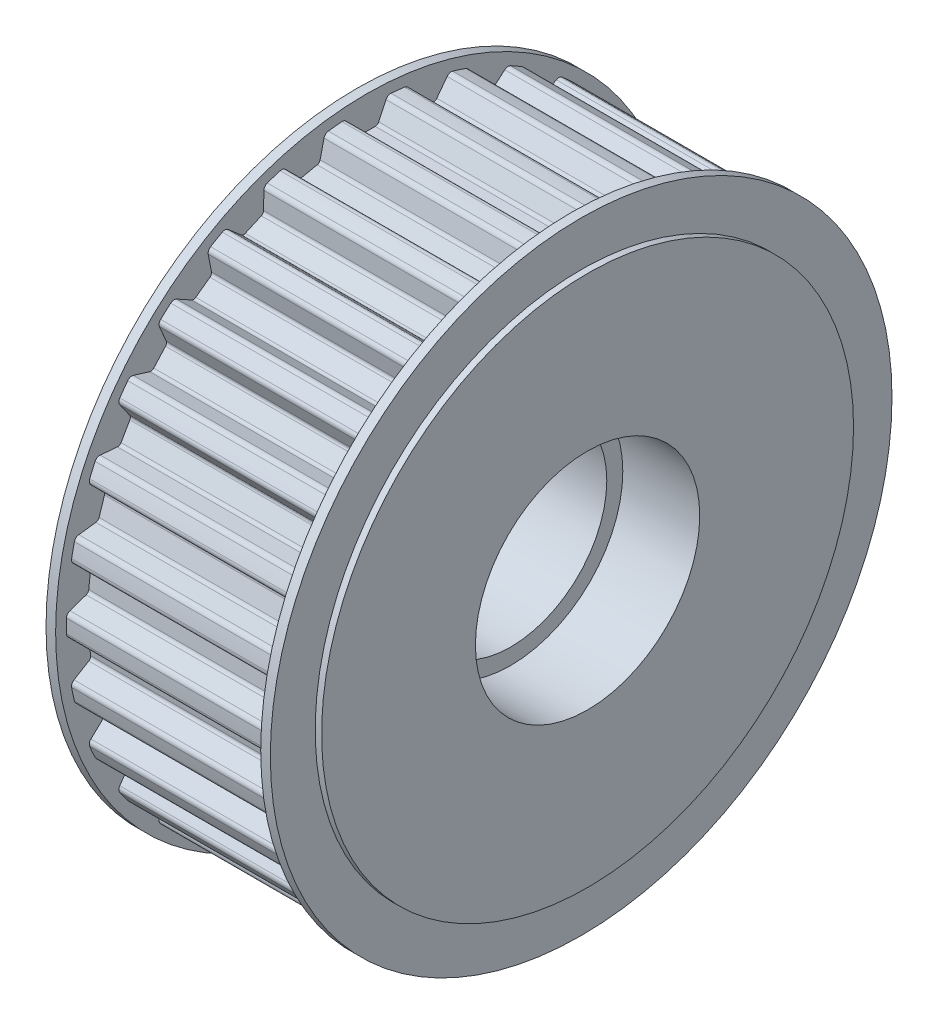
SolidWorks part; units mm, degrees
ref_plane "前视" through (0, 0, 0) normal (0, 0, 1) x (1, 0, 0)
ref_plane "上视" through (0, 0, 0) normal (0, 1, 0) x (1, 0, 0)
ref_plane "右视" through (0, 0, 0) normal (1, 0, 0) x (0, 0, -1)
sketch "草图1" plane through (0, 0, 0) normal (1, 0, 0) x (0, 0, -1)
  line L0 (0, 46.82) -> (0, 47.201) construction
  circle A1 centre (0, 0) radius 46.82
  circle A2 centre (0, 0) radius 47.201 construction
  dimension "D2" = 93.64
  dimension "D3" = 0.381
extrude "拉伸1" add sketch "草图1" along normal mid plane 32
sketch "草图2" plane through (16, 0, 0) normal (1, 0, 0) x (0, 0, -1)
  line L0 (0, 0) -> (0, 61.5267) construction
  line L1 (-3.285, 46.7046) -> (-1.7534, 43.42)
  line L2 (-1.7534, 43.42) -> (1.7534, 43.42)
  line L3 (1.7534, 43.42) -> (3.285, 46.7046)
  circle A0 centre (0, 0) radius 46.82 construction
  arc A1 (3.285, 46.7046) -> (-3.285, 46.7046) centre (0, 0) ccw
  dimension "D2" = 3.4
  dimension "D3" = 25
  dimension "D1" = 6.57
extrude "拉伸2" cut sketch "草图2" against normal up to surface (32 mm away) up to face at (-16, 0, -46.82)
fillet "圆角1" radius 0.6 2 edges at (0, 43.42, -1.7534) (0, 43.42, 1.7534)
fillet "圆角2" radius 0.8 2 edges at (0, 46.7046, -3.285) (0, 46.7046, 3.285)
pattern_circular "阵列(圆周)1" count 30 over 360 about axis through (0, 0, 0) along (1, 0, 0) of "拉伸2", "圆角1", "圆角2"
sketch "草图6" plane through (16, 0, 0) normal (1, 0, 0) x (0, 0, -1)
  circle A0 centre (0, 0) radius 48.5
  dimension "D1" = 97
extrude "凸台-拉伸2" add sketch "草图6" along normal blind 1.5
sketch "草图7" plane through (17.5, 0, 0) normal (1, 0, 0) x (0, 0, -1)
  circle A0 centre (0, 0) radius 41.5
  dimension "D1" = 83
extrude "凸台-拉伸3" add sketch "草图7" along normal blind 1
mirror "镜向2" about plane through (0, 0, 0) normal (1, 0, 0) of "凸台-拉伸3", "凸台-拉伸2"
sketch "草图8" plane through (-18.5, 0, 0) normal (-1, 0, 0) x (0, 0, 1)
  circle A0 centre (0, 0) radius 15
  dimension "D1" = 30
extrude "切除-拉伸1" cut sketch "草图8" against normal through all
sketch "草图9" plane through (-18.5, 0, 0) normal (-1, 0, 0) x (0, 0, 1)
  circle A0 centre (0, 0) radius 17.5
  dimension "D1" = 35
extrude "切除-拉伸2" cut sketch "草图9" against normal blind 12
mirror "镜向3" about plane through (0, 0, 0) normal (1, 0, 0) of "切除-拉伸2"
sketch "草图10" plane through (-18.5, 0, 0) normal (-1, 0, 0) x (0, 0, 1)
  circle A0 centre (0, 0) radius 20
  dimension "D1" = 40
extrude "切除-拉伸3" [suppressed] cut sketch "草图10" against normal blind 2
mirror "镜向4" [suppressed] about plane through (0, 0, 0) normal (1, 0, 0)
